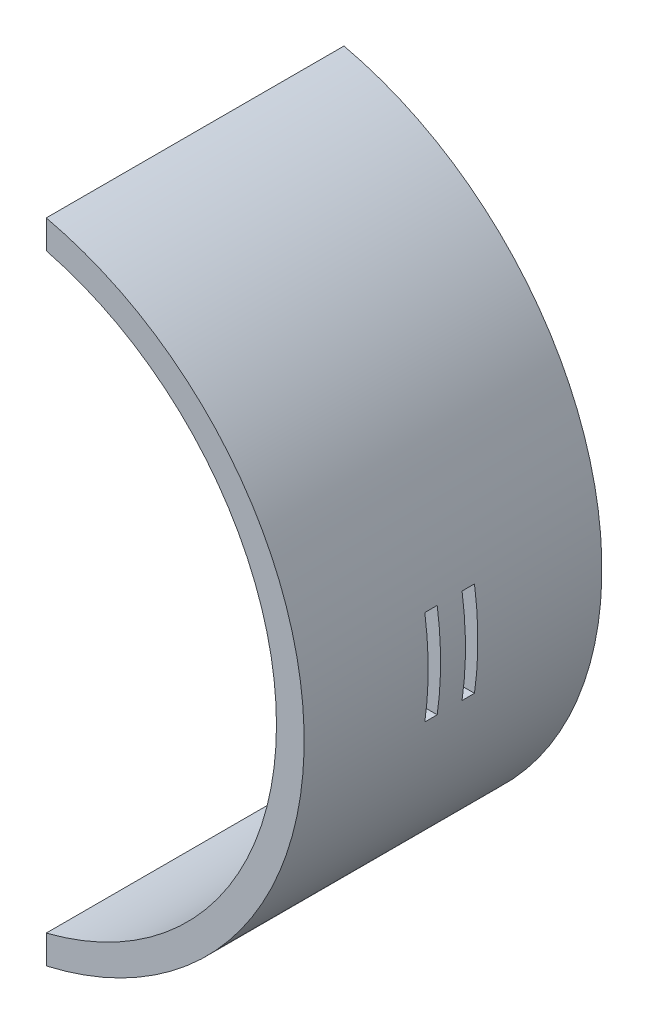
from build123d import *

# Parameters (mm, degrees)
EXTRUDE_1_DEPTH     = 60
SKETCH_3_W          = 2.5
SKETCH_3_H          = 19.1
CUT_EXTRUDE_2_DEPTH = 115


with BuildPart() as part:
    # 草图1 → 凸台-拉伸1 (new body)
    with BuildSketch(Plane.XY):
        with BuildLine():
            Line((15, 65.276254084), (15, 59.535511754))
            ThreePointArc((15, 59.535511754), (61.396067951, 0), (15, -59.535511754))
            Line((15, -59.535511754), (15, -65.276254084))
            ThreePointArc((15, -65.276254084), (66.977528674, 0), (15, 65.276254084))
        make_face()
    extrude(amount=EXTRUDE_1_DEPTH)

    # 草图3 → 切除-拉伸2 (cut)
    with BuildSketch(Plane(origin=(0, 0, 0), x_dir=(0, 0, -1), z_dir=(1, 0, 0))):
        with Locations((-33.75394201, 0)):
            Rectangle(SKETCH_3_W, SKETCH_3_H)
        with Locations((-26.24605799, 0)):
            Rectangle(SKETCH_3_W, SKETCH_3_H)
    extrude(amount=CUT_EXTRUDE_2_DEPTH, mode=Mode.SUBTRACT)


solid = part.part
